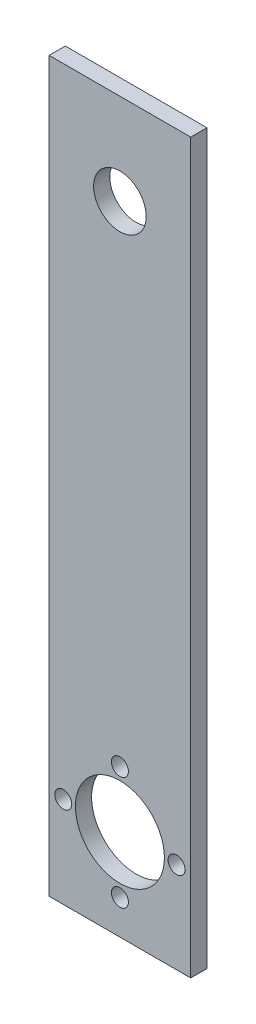
from build123d import *

# Parameters (mm, degrees)
SKETCH1_W           = 35
SKETCH1_H           = 180
SKETCH1_R           = 6.5
SKETCH1_R_2         = 11
BOSS_EXTRUDE1_DEPTH = 4
SKETCH2_R           = 2.1
CUT_EXTRUDE2_DEPTH  = 10


with BuildPart() as part:
    # Sketch1 → Boss-Extrude1 (new body)
    with BuildSketch(Plane.XY):
        with Locations((17.5, -90)):
            Rectangle(SKETCH1_W, SKETCH1_H)
        with Locations((17.5, -22.5)):
            Circle(SKETCH1_R, mode=Mode.SUBTRACT)
        with Locations((17.5, -157.5)):
            Circle(SKETCH1_R_2, mode=Mode.SUBTRACT)
    extrude(amount=BOSS_EXTRUDE1_DEPTH)

    # Sketch2 → Cut-Extrude2 (cut)
    with BuildSketch(Plane.XY.offset(4)):
        with Locations((3.5, -157.5)):
            Circle(SKETCH2_R)
        with Locations((17.5, -143.5)):
            Circle(SKETCH2_R)
        with Locations((31.5, -157.5)):
            Circle(SKETCH2_R)
        with Locations((17.5, -171.5)):
            Circle(SKETCH2_R)
    extrude(amount=-CUT_EXTRUDE2_DEPTH, mode=Mode.SUBTRACT)


solid = part.part
